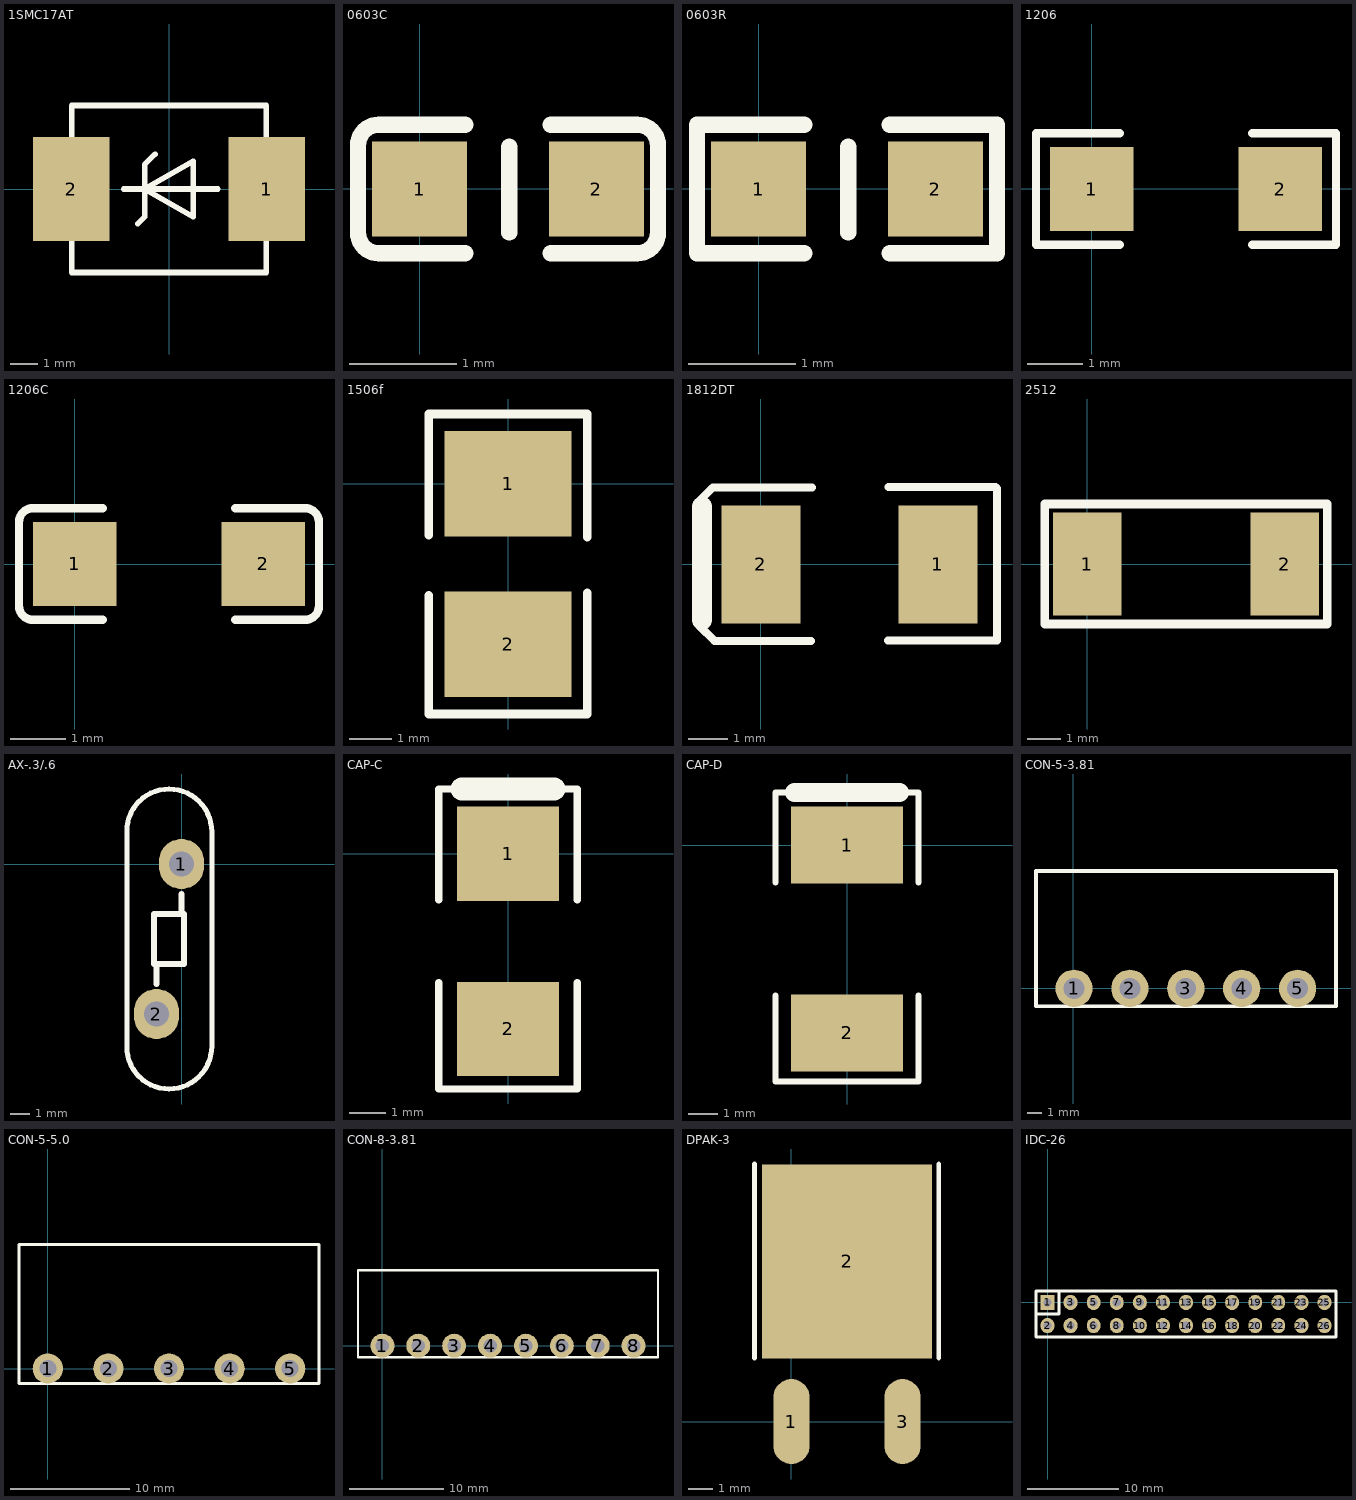
[diagram p0: the footprints below, top view; thin cyan lines are the x and y axes]
# Altium footprint library MISC103926-16.PcbLib: 32 footprints (part 1 of 2)
Each footprint in its own frame and in the unit in brackets; x right, y up, seen from the top. Pads: shape width x height; smd on the part's side, far side on the other; paste and mask are expansions set on the pad; w line width, h text height; cw(c..) or ccw(c..) is an arc to the next point about the centre after c.

## 1SMC17AT [mil]
height 78.74
pads (2):
  rect 110x150 smd: 1(140.5,0) 2(-140.5,0)
Top Overlay:
  lines w8: -140,-40 ccw(c-140,0) -140,40 ; -65,0 -35,0 ; -45,-50 -35,-40 -35,35 -20,50 ; 70,0 -35,0 ; -35,0 35,40 35,-40 -35,0 ; -140,-120 140,-120 140,120 -140,120 -140,-120

## 0603C [mil]
height 270.08
pads (2):
  rect 35x35 smd: 1(0,0) 2(65,0)
Top Overlay:
  lines w6: 16.75,-23.62 -15,-23.62 cw(c-15,-16) -22.62,-16 -22.62,16 cw(c-15,16) -15,23.62 16.75,23.62 ; 33,-16 33,15.5 ; 48.25,-23.62 80,-23.62 ccw(c80,-16) 87.62,-16 87.62,16 ccw(c80,16) 80,23.62 48.25,23.62

## 0603R [mil]
height 270.08
pads (2):
  rect 35x35 smd: 1(0,0) 2(65,0)
Top Overlay:
  lines w6: 16.75,-23.62 -22.62,-23.62 -22.62,23.62 16.75,23.62 ; 33,-16 33,15.49 ; 48.24,-23.62 87.61,-23.62 87.61,23.62 48.24,23.62

## 1206 [mil]
height 270.08
pads (2):
  rect 60x60 smd: 1(0,0) 2(135,0)
Top Overlay:
  lines w6: 20,-40 -40,-40 -40,40 20,40 ; 115,-40 175,-40 175,40 115,40

## 1206C [mil]
height 270.08
pads (2):
  rect 60x60 smd: 1(0,0) 2(135,0)
Top Overlay:
  lines w6: 20,-40 -30,-40 cw(c-30,-30) -40,-30 -40,30 cw(c-30,30) -30,40 20,40 ; 115,-40 165,-40 ccw(c165,-30) 175,-30 175,30 ccw(c165,30) 165,40 115,40

## 1506f [mm]
height 6.86
pads (2):
  rect 3x2.5 smd: 1(0,0) 2(0,-3.81)
Top Overlay:
  lines w0.203: -1.88,-2.642 -1.88,-5.461 1.88,-5.461 1.88,-2.591 ; -1.88,-1.219 -1.88,1.651 1.88,1.651 1.88,-1.27

## 1812DT [mm]
height 6.86
pads (2):
  rect 2x3 smd: 1(4.496,0) 2(0,0)
Top Overlay:
  lines w0.203: -1.626,1.549 -1.224,1.951 -1.021,1.951 1.3,1.951 ; -1.575,-1.549 -1.175,-1.949 -0.961,-1.949 1.277,-1.949 ; 3.556,1.97 3.24,1.97 ; 5.462,1.97 3.24,1.97 ; 5.486,-1.93 3.226,-1.93 ; 3.226,-1.93 5.994,-1.93 ; 3.226,-1.93 5.994,-1.93 ; 3.24,1.97 5.955,1.97 5.994,1.93 5.994,-1.93
  lines w0.508: -1.499,-1.412 -1.499,1.473

## 2512 [mil]
height 270.08
pads (2):
  rect 80x120 smd: 1(0,0) 2(230,0)
Top Overlay:
  lines w10: -50,-70 -50,70 280,70 280,-70 -50,-70

## AX-.3/.6 [mil]
height 374.02
pads (2):
  oval 90x100 hole 50: 1(0,0) 2(-50,-300)
Top Overlay:
  lines w10: -109.45,-365.55 ccw(c-25,-365.55) -25,-450 ccw(c-25,-364.45) 60.55,-364.45 60.55,64.45 ccw(c-25,64.45) -25,150 ccw(c-25,65.55) -109.45,65.55 -109.45,-365.55
  lines w12: -55,-200 -55,-100 5,-100 5,-200 -25,-200 -50,-200 -50,-240 ; 0,-100 0,-60

## CAP-C [mm]
pads (2):
  rect 2.8x2.6 smd: 1(0,0) 2(0,-4.826)
Top Overlay:
  lines w0.2: -1.905,-3.556 -1.905,-6.477 1.905,-6.477 1.905,-3.556 ; -1.905,-1.27 -1.905,1.778 1.905,1.778 1.905,-1.27
  lines w0.635: -1.27,1.778 1.27,1.778

## CAP-D [mm]
height 6.86
pads (2):
  rect 3.8x2.6 smd: 1(0,0) 2(0,-6.35)
Top Overlay:
  lines w0.2: -2.413,-5.08 -2.413,-8.001 2.413,-8.001 2.413,-5.08 ; -2.413,-1.27 -2.413,1.778 ; 2.413,-1.27 2.413,1.778
  lines w0.203: -2.413,1.778 2.413,1.778
  lines w0.635: -1.778,1.778 1.778,1.778

## CON-5-3.81 [mil]
pads (5):
  round 100 hole 56: 1(2,0) 2(152,0) 3(302,0) 4(452,0) 5(602,0)
Top Overlay:
  lines w10: -100,-48 705,-48 705,315 -100,315 -100,-48

## CON-5-5.0 [mil]
pads (5):
  round 100 hole 56: 1(0,0) 2(200,0) 3(400,0) 4(600,0) 5(800,0)
Top Overlay:
  lines w10: -95,-50 -95,410 895,410 895,-50 -95,-50

## CON-8-3.81 [mil]
pads (8):
  round 100 hole 56: 1(0,0) 2(150,0) 3(300,0) 4(450,0) 5(600,0) 6(750,0) 7(900,0) 8(1050,0)
Top Overlay:
  lines w10: -102,-48 -102,315 1152,315 1152,-48 -102,-48

## DPAK-3 [mm]
height 0.965
pads (3):
  oval 1.5x3.5 smd: 1(0,0) 3(4.58,0)
  rect 7x8 smd: 2(2.29,6.604)
Top Overlay:
  lines w0.2: -1.52,2.616 -1.52,10.616 ; 6.075,2.616 6.075,10.616

## IDC-26 [mil]
height 270.08
pads (26):
  rect 60x66 hole 35: 1(0,0)
  oval 60x66 hole 35: 2(0,-100) 3(100,0) 4(100,-100) 5(200,0) 6(200,-100) 7(300,0) 8(300,-100) 9(400,0) 10(400,-100) 11(500,0) 12(500,-100) 13(600,0) 14(600,-100) 15(700,0) 16(700,-100) 17(800,0) 18(800,-100) 19(900,0) 20(900,-100) 21(1000,0) 22(1000,-100) 23(1100,0) 24(1100,-100) 25(1200,0) 26(1200,-100)
Top Overlay:
  lines w12: -50,-50 50,-50 50,50 ; -50,-150 -50,50 1250,50 1250,-150 -50,-150